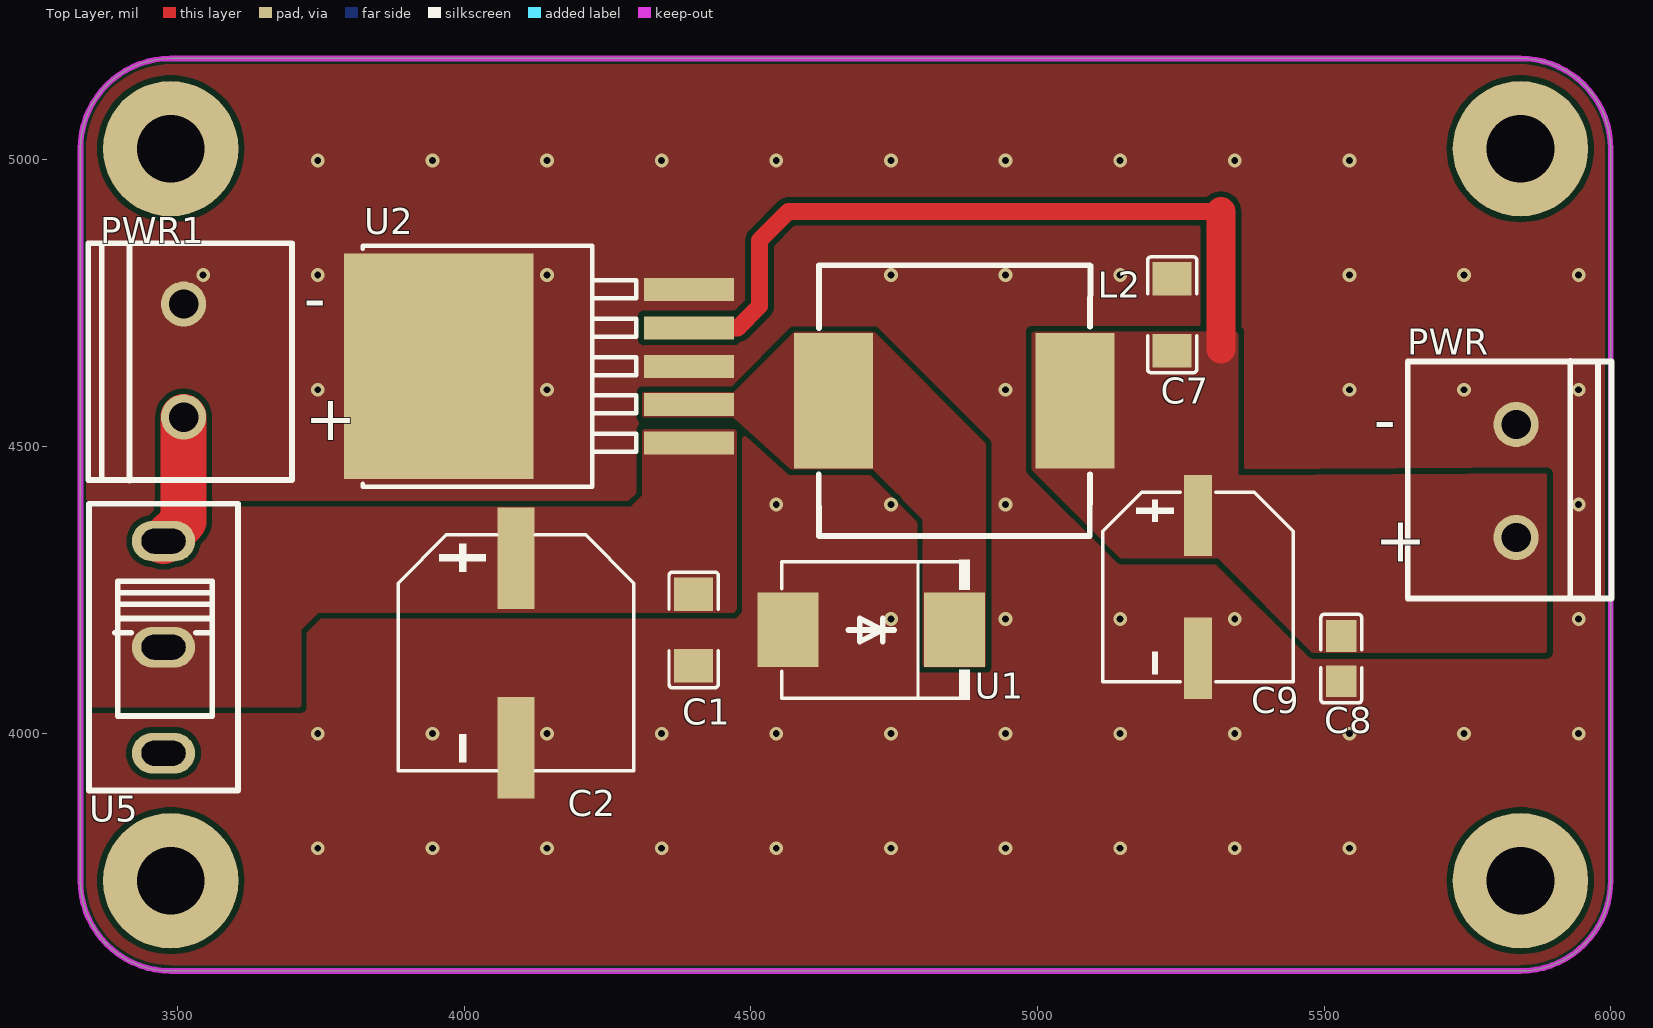
[diagram p0: Top Layer view]
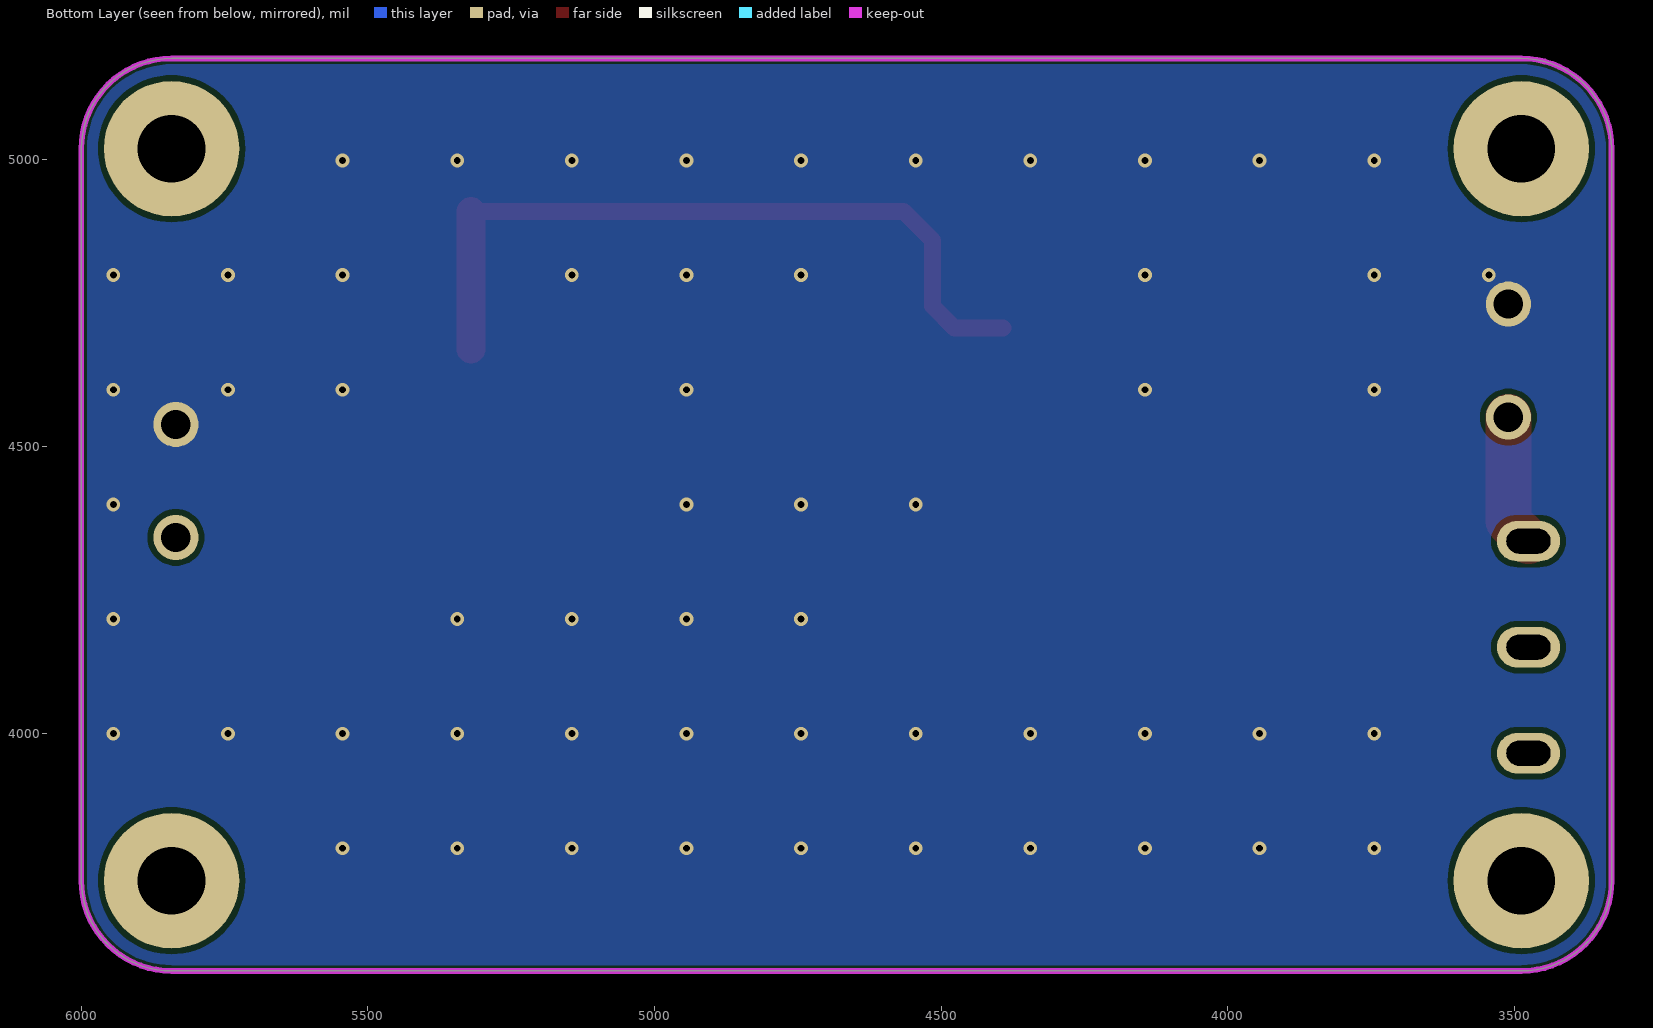
[diagram p1: Bottom Layer view, seen from below]
# Altium PCB MISC49950.pcbdoc
Units mil, origin at the board's own origin, x right, y up, seen from the top; angles counter-clockwise.
Board outline 2670 x 1592.2 mil, 2 copper layers (Top Layer, Bottom Layer), stack 62.206 mil thick; 11 components, 5 nets, 31 pads, 56 vias.

## Layer stack, top to bottom
Top Solder Mask Layer: solder mask 0.394, Dk 3.3
Top Layer: signal copper 1.379
Dielectric1: surface 59.449, FR4, Dk 4.5
Bottom Layer: signal copper 1.378
Bottom Solder Mask Layer: solder mask 0.394, Dk 3.3

## Board outline
3487.48,5177.2 ccw(c3487.48,5019.72) 3330,5019.72 3330,3742.48 ccw(c3487.48,3742.48) 3487.48,3585 5842.52,3585 ccw(c5842.52,3742.48) 6000,3742.48 6000,5019.72 ccw(c5842.52,5019.72) 5842.52,5177.2 3487.48,5177.2

## Design rules (kind name [scope] priority, off if disabled: settings)
BoardOutlineClearance Plane_innerPlane_1 [All] p2 off: genericclearance=6 ignorepadtopadclearanceinfootprint=FALSE except(0: Arc-SplitContinuation Track-SplitContinuation SMDPad-SplitContinuation THPad-SplitContinuation Via-SplitContinuation Fill-SplitContinuation Region-SplitContinuation Poly-SplitContinuation Text-SplitContinuation Hole-SplitContinuation; 6: Arc-CutoutEdge Track-CutoutEdge SMDPad-CutoutEdge THPad-CutoutEdge Via-CutoutEdge Fill-CutoutEdge Region-CutoutEdge Text-CutoutEdge Hole-CutoutEdge; 10: Poly-OutlineEdge Poly-CutoutEdge; 11.8: Arc-OutlineEdge Track-OutlineEdge SMDPad-OutlineEdge THPad-OutlineEdge Via-OutlineEdge Fill-OutlineEdge Region-OutlineEdge Text-OutlineEdge Hole-OutlineEdge)
BoardOutlineClearance Copper_copperRegion_1 [All] p4 off: genericclearance=6 ignorepadtopadclearanceinfootprint=FALSE except(0: Arc-SplitContinuation Track-SplitContinuation SMDPad-SplitContinuation THPad-SplitContinuation Via-SplitContinuation Fill-SplitContinuation Region-SplitContinuation Poly-SplitContinuation Text-SplitContinuation Hole-SplitContinuation; 6: Arc-CutoutEdge Track-CutoutEdge SMDPad-CutoutEdge THPad-CutoutEdge Via-CutoutEdge Fill-CutoutEdge Region-CutoutEdge Text-CutoutEdge Hole-CutoutEdge; 10: Poly-OutlineEdge Poly-CutoutEdge; 11.8: Arc-OutlineEdge Track-OutlineEdge SMDPad-OutlineEdge THPad-OutlineEdge Via-OutlineEdge Fill-OutlineEdge Region-OutlineEdge Text-OutlineEdge Hole-OutlineEdge)
BoardOutlineClearance safeClearance_1 [All] p6: genericclearance=6 ignorepadtopadclearanceinfootprint=FALSE except(0: Arc-SplitContinuation Track-SplitContinuation SMDPad-SplitContinuation THPad-SplitContinuation Via-SplitContinuation Fill-SplitContinuation Region-SplitContinuation Poly-SplitContinuation Text-SplitContinuation Hole-SplitContinuation; 6: Arc-CutoutEdge Track-CutoutEdge SMDPad-CutoutEdge THPad-CutoutEdge Via-CutoutEdge Fill-CutoutEdge Region-CutoutEdge Text-CutoutEdge Hole-CutoutEdge; 10: Poly-OutlineEdge Poly-CutoutEdge; 11.8: Arc-OutlineEdge Track-OutlineEdge SMDPad-OutlineEdge THPad-OutlineEdge Via-OutlineEdge Fill-OutlineEdge Region-OutlineEdge Text-OutlineEdge Hole-OutlineEdge)
Clearance Plane_innerPlane [All] p1 off: gap=6 ignorepadtopadclearanceinfootprint=FALSE except(10: Poly-Track Poly-SMDPad Poly-THPad Poly-Via Poly-Fill Poly-Region Poly-Poly Poly-Arc Poly-Text Poly-Hole)
Clearance Copper_copperRegion [All] p3 off: gap=6 ignorepadtopadclearanceinfootprint=FALSE except(10: Poly-Track Poly-SMDPad Poly-THPad Poly-Via Poly-Fill Poly-Region Poly-Poly Poly-Arc Poly-Text Poly-Hole)
Clearance safeClearance [All] p5: gap=6 ignorepadtopadclearanceinfootprint=FALSE except(10: Poly-Track Poly-SMDPad Poly-THPad Poly-Via Poly-Fill Poly-Region Poly-Poly Poly-Arc Poly-Text Poly-Hole)
DiffPairsRouting differentialPair [All] p1: maxlimit=6 minlimit=6 mostfreqgap=6 toplayer_minwidth=5 toplayer_prefwidth=10 toplayer_maxwidth=100 toplayer_mingap=6 toplayer_prefgap=6 toplayer_maxgap=6 bottomlayer_minwidth=5 bottomlayer_prefwidth=10 bottomlayer_maxwidth=100 bottomlayer_mingap=6 bottomlayer_prefgap=6 bottomlayer_maxgap=6 maxuncoupledlength=10
HoleToHoleClearance otherClearance [All] p1: gap=11.8 allowstackedmicrovias=TRUE
Length netLength [All] p1: minlimit=0 maxlimit=0
PasteMaskExpansion pasteMaskExpansion [All] p1: expansion=0
PlaneConnect innerPlane [All] p1: planeconnectstyle=Relief reliefexpansion=20 reliefentries=4 reliefconductorwidth=10 reliefairgap=10
PolygonConnect copperRegion [All] p1: connectstyle=Direct reliefconductorwidth=10 reliefentries=4 polygonreliefangle="90 Angle" airgapwidth=10 via.connectstyle=Relief via.reliefconductorwidth=10 via.reliefentries=4 via.polygonreliefangle="90 Angle" via.airgapwidth=10
RoutingVias viaSize [All] p1: holewidth=12.01 width=24.02 viastyle="Through Hole" minholewidth=11.81 minwidth=19.68 maxholewidth=236.22 maxwidth=393.7
SolderMaskExpansion solderMaskExpansion [IsVia] p1: expansion=-1000 istentingtop=TRUE
SolderMaskExpansion solderMaskExpansion [All] p2: expansion=2 istentingtop=FALSE
Width trackWidth [All] p1: maxlimit=100 minlimit=5 preferedwidth=10

## Components (designator, comment, footprint, x,y, rotation, side; value= is the part's Value field where it differs from the comment)
C1 "100nF" C1206 4400,4180 r90 top
C2 "220uF" CAP-SMD_BD10.0-L10.3-W10.3-FD-LS11.3 4090,4140 r270 top
C7 "100nF" C1206 5235,4730 r270 top
C8 "10uF" C0805 5530,4130 r90 top
C9 "220uF" CAP-SMD_BD8.0-L8.3-W8.3-FD-1 5280,4255 r270 top
L2 "68uH" IND-SMD_L12.0-W12.0_744771008 4855,4580 r0 top
PWR "CONN-TH_2P-P5.00" CONN-TH_2P-P5.00 5835,4440 r270 top
PWR1 "CONN-TH_2P-P5.00" CONN-TH_2P-P5.00 3510,4650 r90 top
U1 "SS56" SMC_L6.9-W5.9-LS7.9-RD 4710,4180 r180 top
U2 "LM2596HVS-12.0" TO-263-5_L10.0-W8.4-P1.70-LS15.3-BR 4173.51,4640 r0 top
U5 "SS-12D10-G5" SW-TH_SS-12D10-G050 3475,4150 r270 top

## Footprints (in the part's own frame and the unit in brackets; to place one, negate y for a bottom-side part, rotate by r counter-clockwise, add the part's x,y. Pads: shape width x height; smd on the part's side, far side on the other; paste and mask are expansions set on the pad)
C0805 [mm]
  rect 1.41x1.35 smd paste-100 mask+0.051: 1(-1,0) 2(1,0)
  silkscreen extent -1.96,-0.9 1.96,0.9
C1206 [mm]
  rect 1.485x1.728 smd paste-100 mask+0.051: 1(-1.593,0) 2(1.593,0)
  silkscreen extent -2.56,-1.09 2.56,1.09
CAP-SMD_BD8.0-L8.3-W8.3-FD-1 [mm]
  rect 3.61x1.26 smd paste+0 mask+0.051: 1(-3.168,0) 2(3.168,0)
  silkscreen extent -4.2,-4.23 4.2,4.23
CAP-SMD_BD10.0-L10.3-W10.3-FD-LS11.3 [mm]
  rect 4.5x1.65 smd paste+0 mask+0.051: 1(-4.2,0) 2(4.2,0)
  silkscreen extent -5.23,-5.23 5.23,5.23
CONN-TH_2P-P5.00 [mm]
  round 2 hole 1.3 paste+0 mask+0.051: 1(-2.504,0) 2(2.504,0)
  silkscreen extent -5.32,-4.8 5.21,4.23
IND-SMD_L12.0-W12.0_744771008 [mm]
  rect 3.5x6 smd paste+0 mask+0.051: 1(-5.35,0) 2(5.35,0)
  silkscreen extent -6.02,-6 6.03,6
SMC_L6.9-W5.9-LS7.9-RD [mm]
  rect 2.7x3.3 smd paste+0 mask+0.051: 1(-3.686,0) 2(3.686,0)
  silkscreen extent -4.36,-3.1 3.98,3.1
SW-TH_SS-12D10-G050 [mm]
  oval 1.8x2.8 hole 1.1 slot 1.95 at 90 deg paste+0 mask+0.05: 1(-4.7,0) 2(0,0) 3(4.7,0)
  silkscreen extent -6.35,-3.3 6.35,3.3
TO-263-5_L10.0-W8.4-P1.70-LS15.3-BR [mm]
  rect 4x1.02 smd paste+0 mask+0.051: 1(5.55,-3.4) 2(5.55,-1.7) 3(5.55,0) 4(5.55,1.7) 5(5.55,3.4)
  rect 8.4x10 smd paste+0 mask+0.051: 6(-5.55,0)
  silkscreen extent -8.91,-5.33 3.2,5.33

## Free pads (board coordinates)
  round 236.22 hole 118.11: 1(3487.48,3742.48) 2(3487.48,5019.72) 3(5842.52,3742.48) 4(5842.52,5019.72)

## Via types
v1: diameter 24.02, hole 12, Top Layer to Bottom Layer, 56 vias

## Nets (pads, with @x,y where several pads share a name; then routed paths per layer and width w, separated by ;. In a path a pad name is that pad's centre, name@x,y a point inside that pad or via, vN(x,y) a via of type N, cw(c..) or ccw(c..) an arc to the next point about the centre after c; other vN are vias at no path point)
$1N2845: L2.1 U1.1 U2.2
$1N6190: PWR1.1 U5.1 | length 230.9
  Top Layer w80: U5.1 3510,4370.04 PWR1.1
+12V: C7.2 C8.2 C9.1 L2.2 PWR.2 U2.4 | length 1319.5
  Top Layer w29.53: U2.4 4476.93,4706.93 4515,4745 4515,4860 4565,4910 5320,4910
  Top Layer w50: 5320,4670 5320,4910
GND: C1.1 C2.2 C7.1 C8.1 C9.2 PWR1.2 PWR.1 U1.2 U2.3 U2.5 U2.6
  other v1: 3744.1,3799.1 3944.1,3799.1 4144.1,3799.1 4344.1,3799.1 4544.1,3799.1 4744.1,3799.1 4944.1,3799.1 5144.1,3799.1 5344.1,3799.1 5544.1,3799.1 3744.1,3999.1 3944.1,3999.1 4144.1,3999.1 4344.1,3999.1 4544.1,3999.1 4744.1,3999.1 4944.1,3999.1 5144.1,3999.1 5344.1,3999.1 5544.1,3999.1 5744.1,3999.1 5944.1,3999.1 4744.1,4199.1 4944.1,4199.1 5144.1,4199.1 5344.1,4199.1 5944.1,4199.1 4544.1,4399.1 4744.1,4399.1 4944.1,4399.1 5944.1,4399.1 3744.1,4599.1 4144.1,4599.1 4944.1,4599.1 5544.1,4599.1 5744.1,4599.1 5944.1,4599.1 3544.1,4799.1 3744.1,4799.1 4144.1,4799.1 4744.1,4799.1 4944.1,4799.1 5144.1,4799.1 5544.1,4799.1 5744.1,4799.1 5944.1,4799.1 3744.1,4999.1 3944.1,4999.1 4144.1,4999.1 4344.1,4999.1 4544.1,4999.1 4744.1,4999.1 4944.1,4999.1 5144.1,4999.1 5344.1,4999.1 5544.1,4999.1
VCC: C1.2 C2.1 U2.1 U5.2
pads on no net: U5.3

## Polygon pours and split planes (outlines as drawn)
VCC on Top Layer (solid, remove dead copper, pour order 0): 3335,4045 3335,4390 3330,4395 4290,4395 4310,4415 4310,4530 4475,4530 4475,4215 4470,4210 3745,4210 3715,4180 3715,4045
$1N2845 on Top Layer (solid, remove dead copper, pour order 2): 4310,4595 4470,4595 4575,4700 4715,4700 4715,4460 4570,4460 4470,4550 4310,4551
$1N2845 on Top Layer (solid, remove dead copper, pour order 4): 4710,4700 4715,4700 4910,4505 4910,4115 4800,4115 4800,4372.34 4710,4462.34
GND on Bottom Layer (solid, remove dead copper, pour order 10): 3035,5600 3035,3105 6350,3105 6350,5600
GND on Top Layer (solid, remove dead copper, pour order 8): 3000,5530 3000,3000 6400,3000 6400,5530
+12V on Top Layer (solid, remove dead copper, pour order 6): 4990,4700 5350,4700 5350,4449.86 5888.71,4453.65 5888.71,4140 5480,4140 5315,4305 5145,4305 4990,4460

## Keep-outs
Board Outline Layer:
  the board outline again, w10

## Silkscreen, mask and mechanical layers (free items; w line width, h text height)
Top Silkscreen Layer:
  text "-" at 3720,4720 h78.74
  text "+" at 3721.3,4510.63 h78.74
  text "-" at 5586.72,4508.4 h78.74
  text "+" at 5588.01,4299.03 h78.74